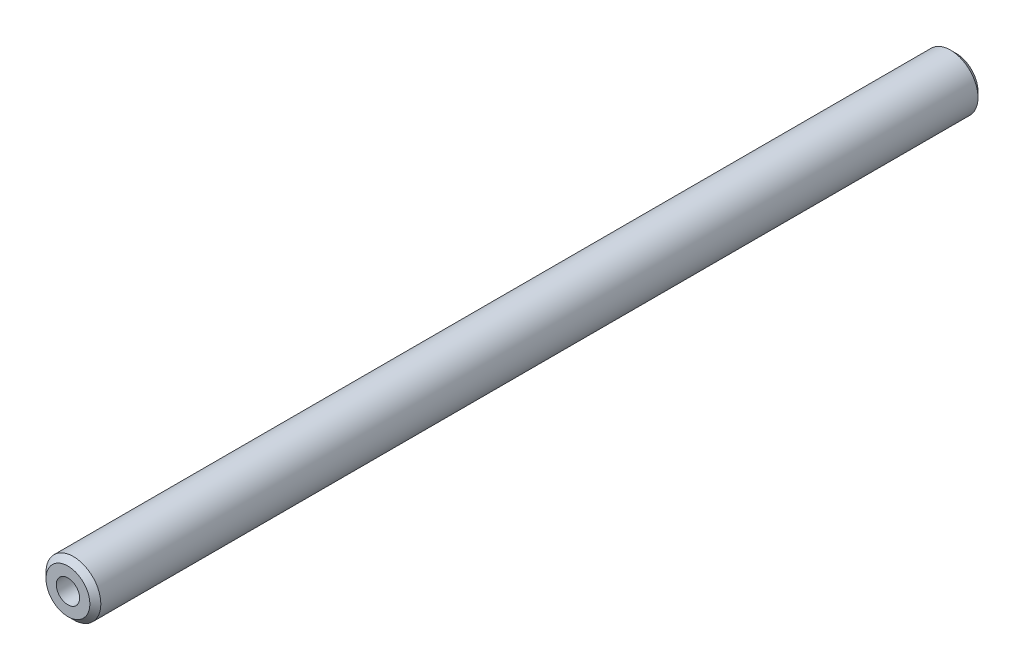
SolidWorks part; units mm, degrees
ref_plane "前视基准面" through (0, 0, 0) normal (0, 0, 1) x (1, 0, 0)
ref_plane "上视基准面" through (0, 0, 0) normal (0, 1, 0) x (1, 0, 0)
ref_plane "右视基准面" through (0, 0, 0) normal (1, 0, 0) x (0, 0, -1)
sketch "草图1" plane through (0, 0, 0) normal (0, 0, 1) x (1, 0, 0)
  circle A0 centre (0, 0) radius 10
  dimension "D1" = 20
extrude "凸台-拉伸1" add sketch "草图1" along normal mid plane 324
chamfer "倒角1" distance 2 angle 45 2 edges at (10, 0, -162) (10, 0, 162)
hole_wizard "M10 螺纹孔1" positions "草图3" profile "草图2" tap size "M10" standard "Gb"
sketch "草图3" plane through (0, 0, 162) normal (0, 0, 1) x (1, 0, 0)
  point P0 (0, 0)
sketch "草图2" plane through (0, 0, 162) normal (1, 0, 0) x (0, -1, 0)
  line L0 (0, 0) -> (0, 27.5537)
  line L1 (0, 27.5537) -> (4.25, 25)
  line L2 (4.25, 25) -> (4.25, 0)
  line L5 (4.25, 0) -> (0, 0)
  line L10 (0, 27.5537) -> (-4.25, 25) construction
  line L11 (0, -6.35) -> (0, 107.95) construction
  dimension "螺纹孔钻头直径" = 8.5
  dimension "螺纹孔钻头深度" = 25
  dimension "导头角度" = 118
hole_wizard "M10 螺纹孔2" positions "草图5" profile "草图4" tap size "M10" standard "Gb"
sketch "草图5" plane through (0, 0, -162) normal (0, 0, -1) x (-1, 0, 0)
  point P0 (0, 0)
sketch "草图4" plane through (0, 0, -162) normal (1, 0, 0) x (0, 1, 0)
  line L0 (0, 0) -> (0, 27.5537)
  line L1 (0, 27.5537) -> (4.25, 25)
  line L2 (4.25, 25) -> (4.25, 0)
  line L5 (4.25, 0) -> (0, 0)
  line L10 (0, 27.5537) -> (-4.25, 25) construction
  line L11 (0, -6.35) -> (0, 107.95) construction
  dimension "螺纹孔钻头直径" = 8.5
  dimension "螺纹孔钻头深度" = 25
  dimension "导头角度" = 118
